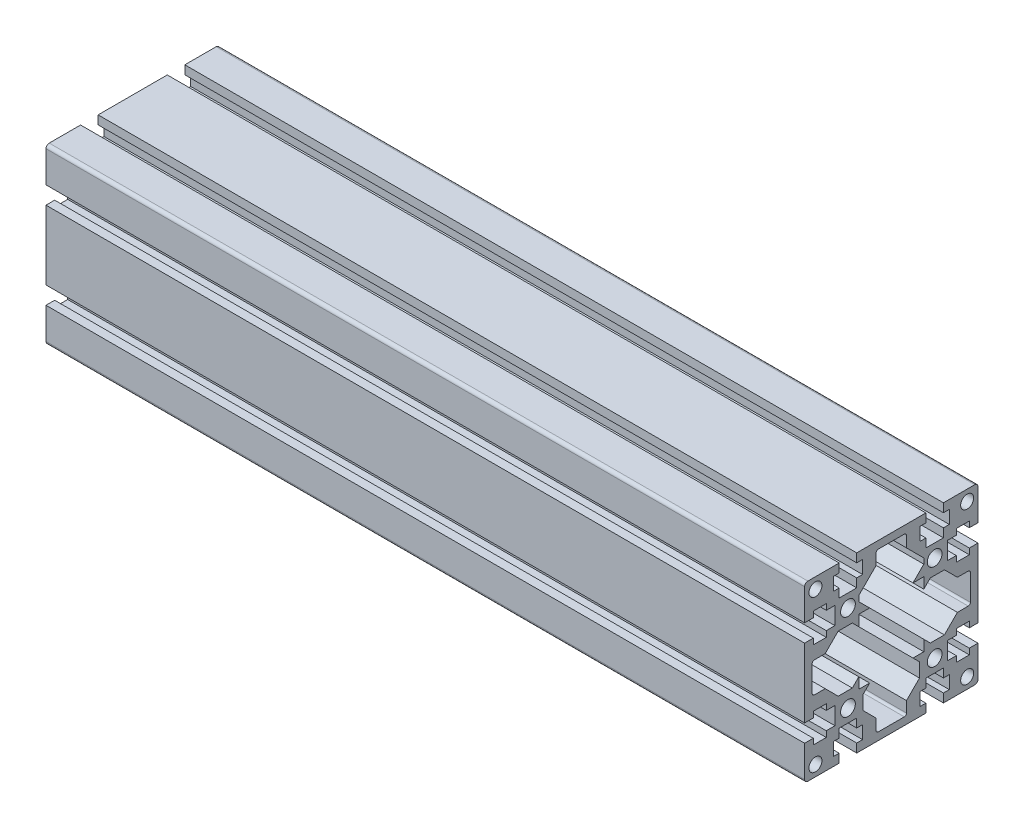
SolidWorks part; units mm, degrees
ref_plane "Front Plane" through (0, 0, 0) normal (0, 0, 1) x (1, 0, 0)
ref_plane "Top Plane" through (0, 0, 0) normal (0, 1, 0) x (1, 0, 0)
ref_plane "Right Plane" through (0, 0, 0) normal (1, 0, 0) x (0, 0, -1)
sketch "草图1" plane through (0, 0, 0) normal (0, 0, 1) x (1, 0, 0)
  line L0 (-530.3448, 0) -> (-180.3448, 0)
  dimension "D1" = 350
other "Aluminium profile 80 X 80G X R1.5(1)"
ref_plane "Plane2" through (-530.3448, 0, 0) normal (1, 0, 0) x (0, 1, 0)
sketch "Sketch1" plane through (-530.3448, 0, 0) normal (1, 0, 0) x (0, 1, 0)
  line L0 (0, 40) -> (0, 0) construction
  line L1 (0, 0) -> (40, 0) construction
  line L2 (-24.05, 40) -> (-24.05, 36)
  line L3 (-38.5, 40) -> (-24.05, 40)
  line L4 (-40, 38.5) -> (-40, 24.05)
  line L5 (-38.5, -40) -> (-24.05, -40)
  line L6 (40, 38.5) -> (40, 24.05)
  line L7 (-24.05, 36) -> (-26.75, 36)
  line L8 (-26.75, 36) -> (-26.75, 30)
  line L9 (-26.75, 30) -> (-24.05, 30)
  line L10 (-24.05, 30) -> (-24.05, 26)
  line L11 (-24.05, 26) -> (-15.95, 26)
  line L12 (-15.95, 26) -> (-15.95, 30)
  line L13 (-15.95, 30) -> (-13.25, 30)
  line L14 (-13.25, 30) -> (-13.25, 36)
  line L15 (-13.25, 36) -> (-15.95, 36)
  line L16 (-15.95, 36) -> (-15.95, 40)
  line L17 (-40, 15.95) -> (-36, 15.95)
  line L18 (-36, 15.95) -> (-36, 13.25)
  line L19 (-15.95, 40) -> (15.95, 40)
  line L20 (-20, 20) -> (-20, 40) construction
  line L21 (20, 20) -> (20, 40) construction
  line L22 (15.95, 36) -> (15.95, 40)
  line L23 (13.25, 36) -> (15.95, 36)
  line L24 (13.25, 30) -> (13.25, 36)
  line L25 (15.95, 30) -> (13.25, 30)
  line L26 (-36, 13.25) -> (-30, 13.25)
  line L27 (-30, 13.25) -> (-30, 15.95)
  line L28 (-26, 15.95) -> (-26, 24.05)
  line L29 (-26, 24.05) -> (-30, 24.05)
  line L30 (-30, 24.05) -> (-30, 26.75)
  line L31 (-30, 26.75) -> (-36, 26.75)
  line L32 (-36, 26.75) -> (-36, 24.05)
  line L33 (-36, 24.05) -> (-40, 24.05)
  line L34 (-30, 15.95) -> (-26, 15.95)
  line L35 (15.95, 26) -> (15.95, 30)
  line L36 (24.05, 26) -> (15.95, 26)
  line L37 (24.05, 30) -> (24.05, 26)
  line L38 (26.75, 30) -> (24.05, 30)
  line L39 (26.75, 36) -> (26.75, 30)
  line L40 (24.05, 36) -> (26.75, 36)
  line L41 (24.05, 40) -> (24.05, 36)
  line L42 (24.05, -40) -> (24.05, -36)
  line L43 (24.05, -36) -> (26.75, -36)
  line L44 (26.75, -36) -> (26.75, -30)
  line L45 (26.75, -30) -> (24.05, -30)
  line L46 (24.05, -30) -> (24.05, -26)
  line L47 (24.05, -26) -> (15.95, -26)
  line L48 (15.95, -26) -> (15.95, -30)
  line L49 (15.95, -30) -> (13.25, -30)
  line L50 (13.25, -30) -> (13.25, -36)
  line L51 (13.25, -36) -> (15.95, -36)
  line L52 (15.95, -36) -> (15.95, -40)
  line L53 (-15.95, -36) -> (-15.95, -40)
  line L54 (-13.25, -36) -> (-15.95, -36)
  line L55 (-13.25, -30) -> (-13.25, -36)
  line L56 (-15.95, -30) -> (-13.25, -30)
  line L57 (-15.95, -26) -> (-15.95, -30)
  line L58 (-24.05, -26) -> (-15.95, -26)
  line L59 (-24.05, -30) -> (-24.05, -26)
  line L60 (-26.75, -30) -> (-24.05, -30)
  line L61 (-26.75, -36) -> (-26.75, -30)
  line L62 (-24.05, -36) -> (-26.75, -36)
  line L63 (-24.05, -40) -> (-24.05, -36)
  line L64 (-30, -15.95) -> (-26, -15.95)
  line L65 (-36, -26.75) -> (-36, -24.05)
  line L66 (-30, -26.75) -> (-36, -26.75)
  line L67 (-30, -24.05) -> (-30, -26.75)
  line L68 (-26, -24.05) -> (-30, -24.05)
  line L69 (-26, -15.95) -> (-26, -24.05)
  line L70 (-30, -13.25) -> (-30, -15.95)
  line L71 (-36, -13.25) -> (-30, -13.25)
  line L72 (-36, -15.95) -> (-36, -13.25)
  line L73 (36, 24.05) -> (40, 24.05)
  line L74 (40, 15.95) -> (36, 15.95)
  line L75 (36, -15.95) -> (36, -13.25)
  line L76 (36, -13.25) -> (30, -13.25)
  line L77 (30, -13.25) -> (30, -15.95)
  line L78 (26, -15.95) -> (26, -24.05)
  line L79 (26, -24.05) -> (30, -24.05)
  line L80 (30, -24.05) -> (30, -26.75)
  line L81 (30, -26.75) -> (36, -26.75)
  line L82 (36, -26.75) -> (36, -24.05)
  line L83 (30, -15.95) -> (26, -15.95)
  line L84 (30, 15.95) -> (26, 15.95)
  line L85 (36, 26.75) -> (36, 24.05)
  line L86 (30, 26.75) -> (36, 26.75)
  line L87 (30, 24.05) -> (30, 26.75)
  line L88 (26, 24.05) -> (30, 24.05)
  line L89 (26, 15.95) -> (26, 24.05)
  line L90 (30, 13.25) -> (30, 15.95)
  line L91 (36, 13.25) -> (30, 13.25)
  line L92 (36, 15.95) -> (36, 13.25)
  line L93 (-36, -15.95) -> (-40, -15.95)
  line L94 (-36, -24.05) -> (-40, -24.05)
  line L95 (36, -15.95) -> (40, -15.95)
  line L96 (36, -24.05) -> (40, -24.05)
  line L97 (-13, 18) -> (-10, 15)
  line L98 (-15, 15) -> (-10, 15)
  line L99 (-15, 15) -> (-15, 10)
  line L100 (-15, -15) -> (-10, -15)
  line L101 (15, 15) -> (15, 10)
  line L102 (-18, 13) -> (-15, 10)
  line L104 (13, 18) -> (10, 15)
  line L105 (13, -18) -> (10, -15)
  line L106 (20, -15) -> (15, -10)
  line L107 (-18, -13) -> (-15, -10)
  line L108 (-13, -18) -> (-10, -15)
  line L109 (15, -10) -> (15, -15)
  line L110 (10, 15) -> (15, 15)
  line L111 (-15, -10) -> (-15, -15)
  line L112 (10, -15) -> (15, -15)
  line L113 (15, 10) -> (20, 15)
  line L235 (24.05, 40) -> (38.5, 40)
  line L249 (-40, 15.95) -> (-40, -15.95)
  line L250 (-20, 20) -> (-26, 20) construction
  line L264 (40, 15.95) -> (40, -15.95)
  line L265 (-13, 24.5) -> (-7, 30.5)
  line L266 (-7, 30.5) -> (-7, 35.5)
  line L267 (7, 35.5) -> (7, 30.5)
  line L268 (7, 30.5) -> (13, 24.5)
  line L269 (-6, -36.5) -> (6, -36.5)
  line L270 (-13, 24.5) -> (-13, 18)
  line L271 (-35.5, 7) -> (-30.5, 7)
  line L272 (-30.5, 7) -> (-24.5, 13)
  line L273 (-24.5, 13) -> (-18, 13)
  line L274 (13, 24.5) -> (13, 18)
  line L275 (-15.95, -40) -> (15.95, -40)
  line L276 (35.5, 7) -> (30.5, 7)
  line L277 (30.5, 7) -> (22.5, 15)
  line L278 (24.05, -40) -> (38.5, -40)
  line L279 (20, 15) -> (22.5, 15)
  line L333 (-13, -24.5) -> (-13, -18)
  line L336 (-13, -24.5) -> (-7, -30.5)
  line L385 (-7, -30.5) -> (-7, -35.5)
  line L386 (-36.5, 6) -> (-36.5, -6)
  line L387 (7, -35.5) -> (7, -30.5)
  line L429 (7, -30.5) -> (13, -24.5)
  line L430 (13, -24.5) -> (13, -18)
  line L494 (20, -15) -> (22.5, -15)
  line L496 (30.5, -7) -> (22.5, -15)
  line L497 (35.5, -7) -> (30.5, -7)
  line L498 (-24.5, -13) -> (-18, -13)
  line L499 (-30.5, -7) -> (-24.5, -13)
  line L500 (-35.5, -7) -> (-30.5, -7)
  line L512 (40, -24.05) -> (40, -38.5)
  line L519 (-40, -24.05) -> (-40, -38.5)
  line L520 (-6, 36.5) -> (6, 36.5)
  line L523 (36.5, 6) -> (36.5, -6)
  circle A0 centre (-20, 20) radius 3.4
  circle A2 centre (20, 20) radius 3.4
  circle A3 centre (20, -20) radius 3.4
  circle A7 centre (-20, -20) radius 3.4
  arc A8 (-38.5, 40) -> (-40, 38.5) centre (-38.5, 38.5) ccw
  arc A9 (-40, -38.5) -> (-38.5, -40) centre (-38.5, -38.5) ccw
  arc A10 (38.5, -40) -> (40, -38.5) centre (38.5, -38.5) ccw
  arc A11 (38.5, 40) -> (40, 38.5) centre (38.5, 38.5) cw
  circle A12 centre (-35, 35) radius 3
  circle A13 centre (35, 35) radius 3
  circle A14 centre (35, -35) radius 3
  arc A15 (-6, 36.5) -> (-7, 35.5) centre (-6, 35.5) ccw
  arc A16 (6, 36.5) -> (7, 35.5) centre (6, 35.5) cw
  arc A17 (-36.5, 6) -> (-35.5, 7) centre (-35.5, 6) cw
  arc A18 (-36.5, -6) -> (-35.5, -7) centre (-35.5, -6) ccw
  arc A19 (36.5, -6) -> (35.5, -7) centre (35.5, -6) cw
  arc A20 (36.5, 6) -> (35.5, 7) centre (35.5, 6) ccw
  arc A21 (6, -36.5) -> (7, -35.5) centre (6, -35.5) ccw
  arc A22 (-6, -36.5) -> (-7, -35.5) centre (-6, -35.5) cw
  point P48 (-20, 20)
  point P97 (0, 0)
  point P104 (-7, 36.5)
  point P185 (40, 40)
  point P187 (40, -40)
  point P188 (-40, -40)
  point P190 (-40, 40)
  dimension "D1" = 80
  dimension "D2" = 80
  dimension "D3" = 20
  dimension "D4" = 8.1
  dimension "D5" = 45
  dimension "D6" = 7
  dimension "D7" = 13.5
  dimension "D8" = 6
  dimension "D12" = 5
  dimension "D13" = 5
  dimension "D14" = 20
  dimension "D18" = 1
  dimension "D19" = 14
  dimension "D15" = 6.8
  dimension "D27" = 45
  dimension "D20" = 1.5
  dimension "D11" = 6
  dimension "D9" = 4
  dimension "D10" = 14
  dimension "D16" = 14
  dimension "D17" = 45
  dimension "D21" = 3.5
  dimension "D22" = 3.5
  dimension "D23" = 73
  dimension "D24" = 30
  dimension "D25" = 30
  dimension "D26" = 45
  dimension "D28" = 5
sketch "Sketch10" plane through (-180.3448, 0, 0) normal (1, 0, 0) x (0, 0, -1)
  circle A0 centre (35, -35) radius 3
  circle A1 centre (-35, -35) radius 3 construction
  circle A2 centre (35, 35) radius 3 construction
  dimension "D1" = 6
  dimension "D2" = 70
  dimension "D3" = 70
extrude "Cut-Extrude1" cut sketch "Sketch10" against normal through all
